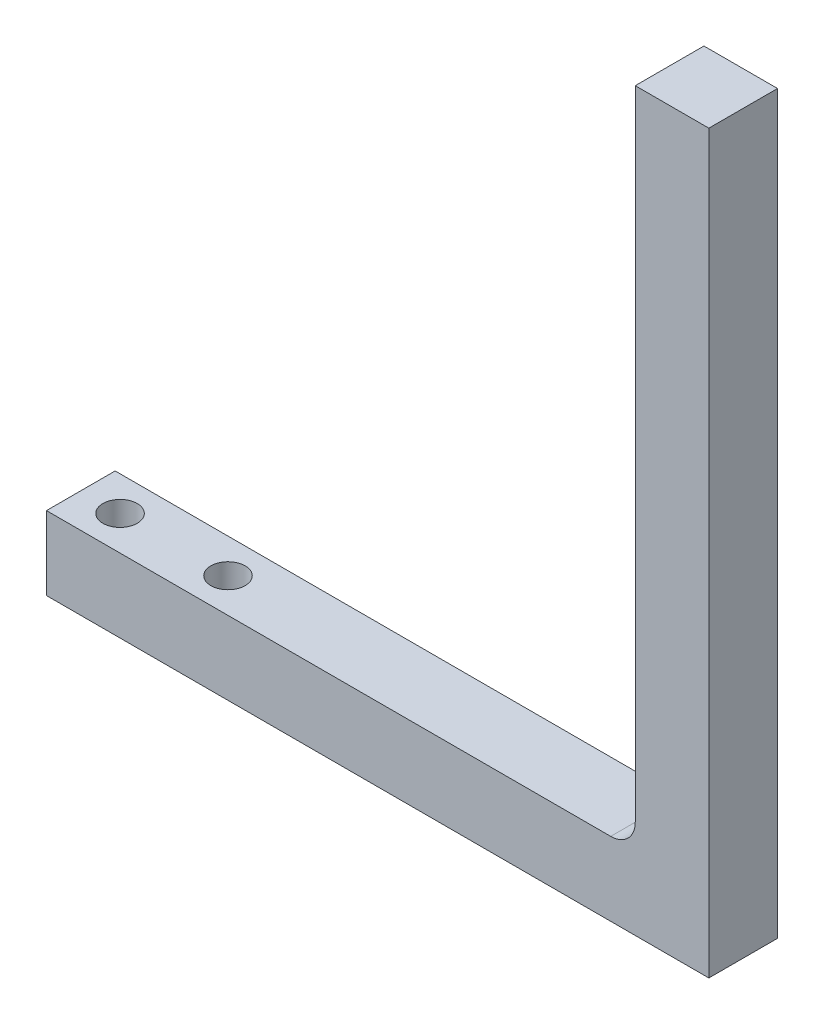
SolidWorks part; units mm, degrees
ref_plane "前视基准面" through (0, 0, 0) normal (0, 0, 1) x (1, 0, 0)
ref_plane "上视基准面" through (0, 0, 0) normal (0, 1, 0) x (1, 0, 0)
ref_plane "右视基准面" through (0, 0, 0) normal (1, 0, 0) x (0, 0, -1)
sketch "草图1" plane through (0, 0, 0) normal (0, 0, 1) x (1, 0, 0)
  line L0 (0, 150) -> (-15, 150)
  line L1 (-15, 150) -> (-15, 15)
  line L2 (-15, 15) -> (-135, 15)
  line L3 (-135, 15) -> (-135, 0)
  line L5 (0, 150) -> (0, 0)
  line L8 (0, 0) -> (-135, 0)
  dimension "D1" = 15
  dimension "D2" = 15
  dimension "D3" = 135
  dimension "D4" = 150
extrude "凸台-拉伸1" add sketch "草图1" along normal mid plane 14
fillet "圆角1" radius 5
sketch "草图3" plane through (0, 15, 0) normal (0, 1, 0) x (1, 0, 0)
  line L0 (-135, -7) -> (-135, 7) construction
  circle A0 centre (-127, 0) radius 3.5
  circle A1 centre (-105, 0) radius 3.5
  dimension "D1" = 7
  dimension "D2" = 22
  dimension "D3" = 8
extrude "切除-拉伸1" cut sketch "草图3" against normal up to next
